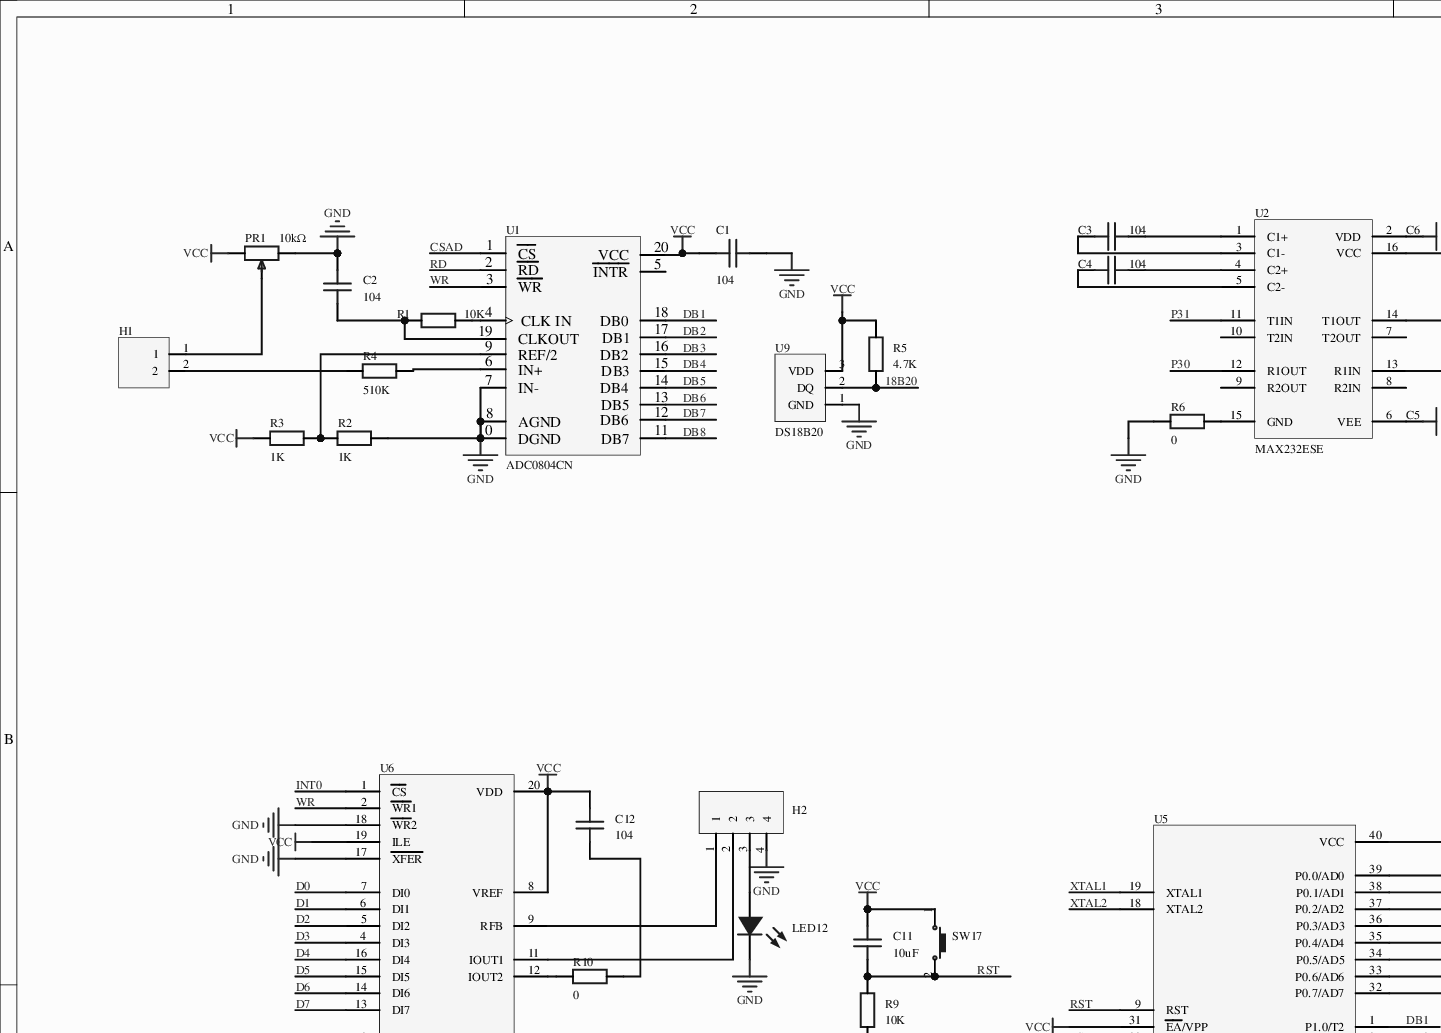
[diagram p0: MISC51981-3.schdoc, top left]
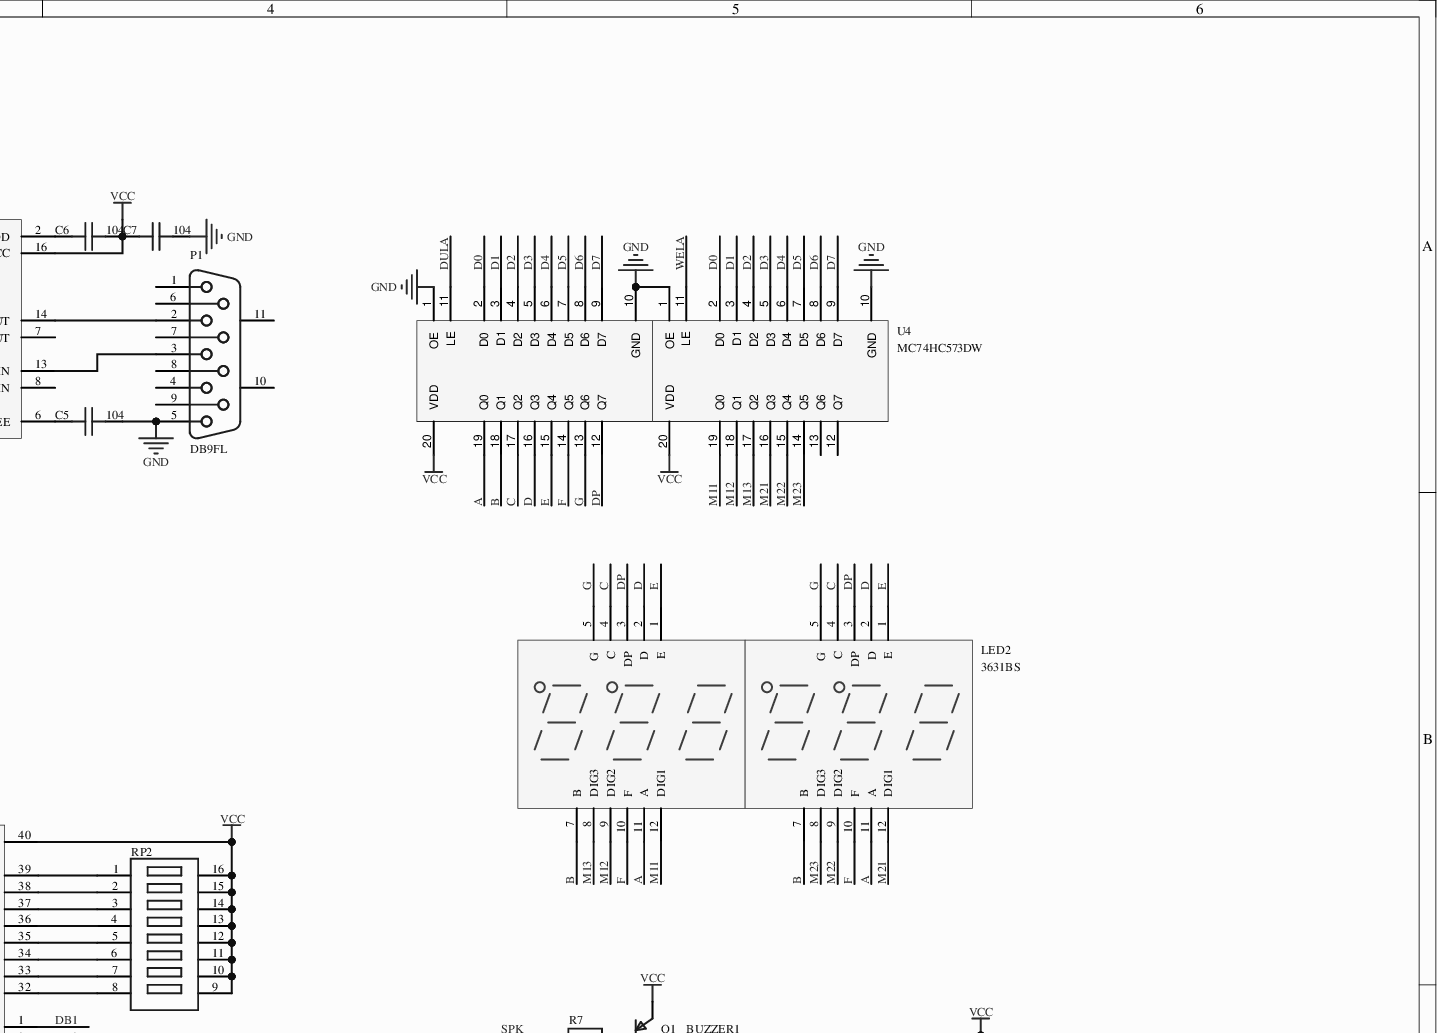
[diagram p1: MISC51981-3.schdoc, top right]
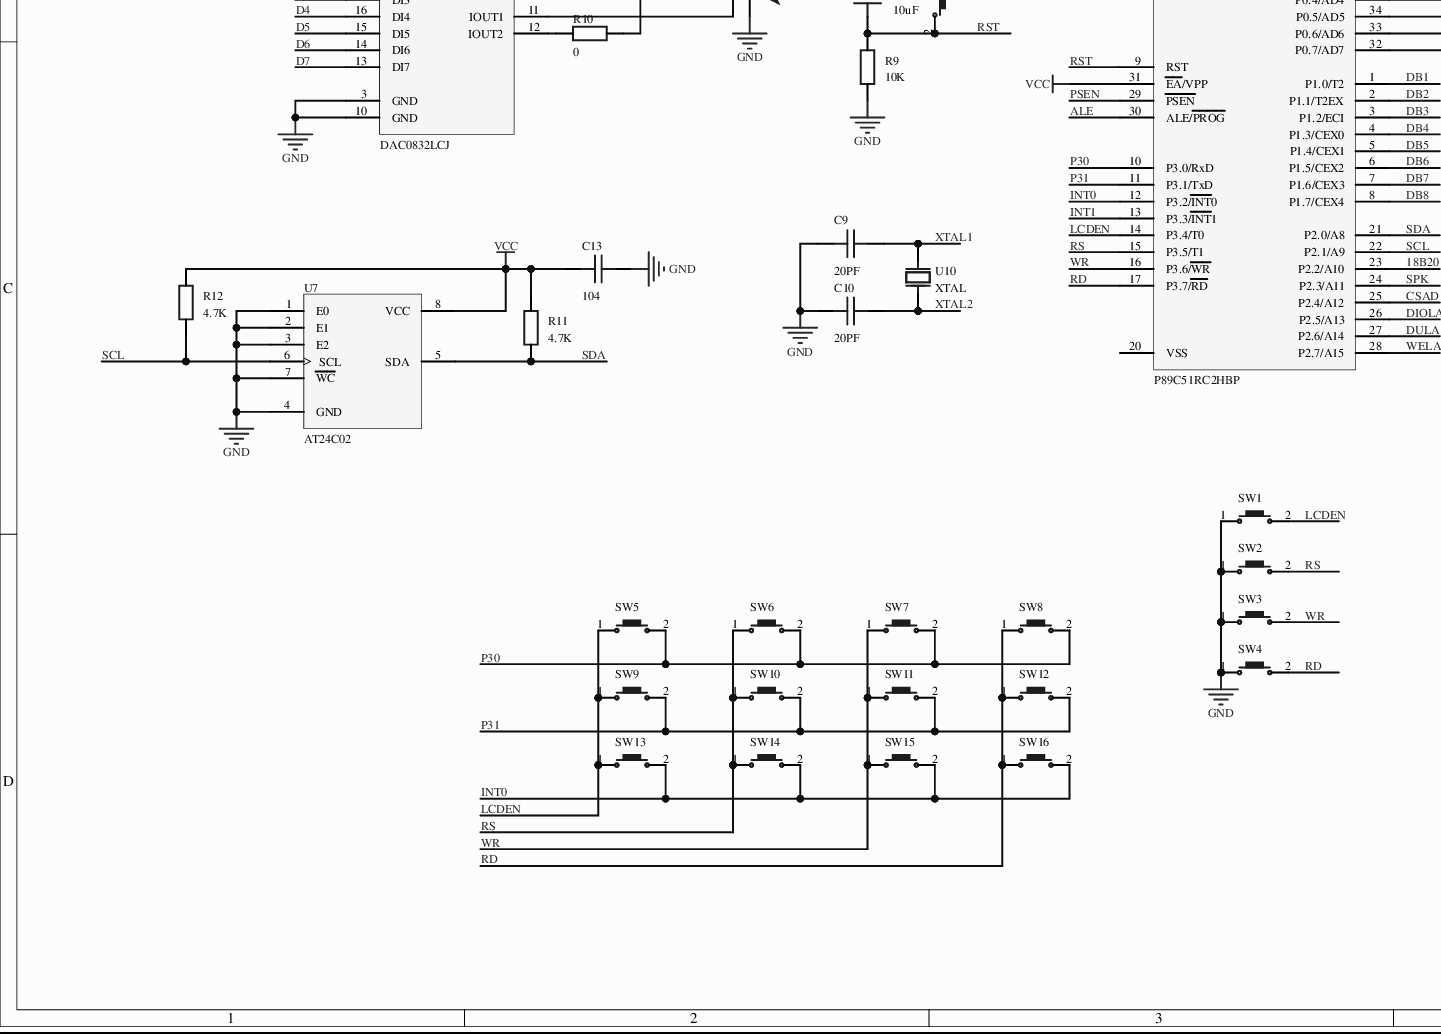
[diagram p2: MISC51981-3.schdoc, bottom left]
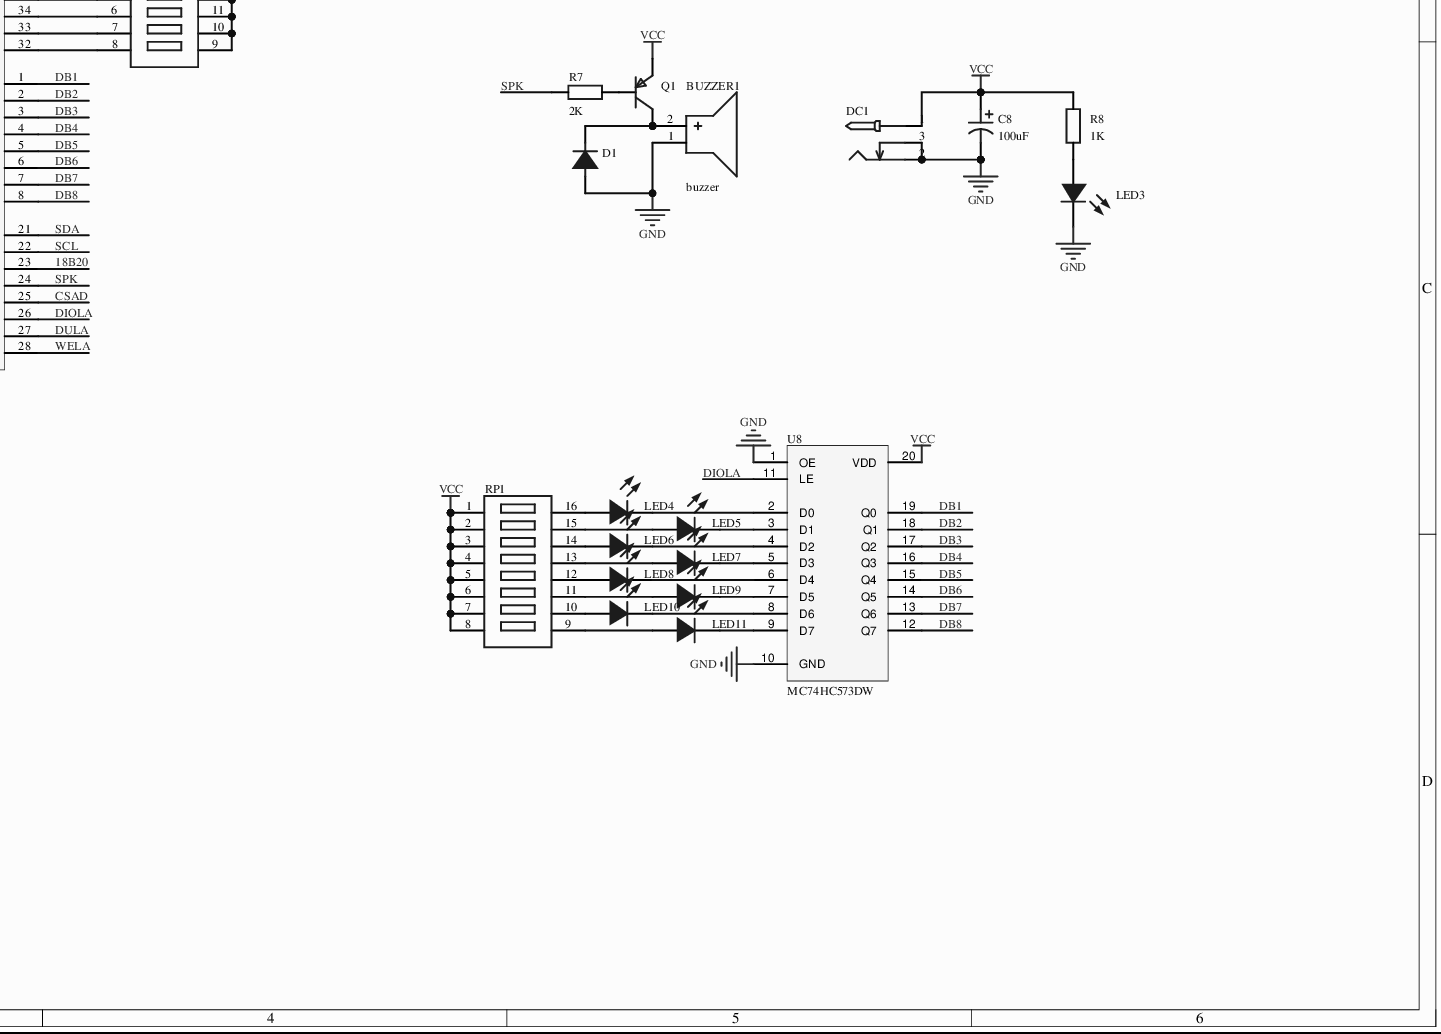
[diagram p3: MISC51981-3.schdoc, bottom right]
# Altium project MISC51981-2.PrjPcb
1 sheet, 74 parts. Net scope: global (net labels, ports and power ports of the same name join across sheets).
Board file: MISC51981.pcbdoc

## Sheet MISC51981-3.schdoc
size 420 x 297 mm; Version: V1.0; @Project Name: MISC51981; @Update Date: 2026-09-29; @Create Date: 2026-09-29; @Board Name: MISC51981; @Create Time: 10:53:11; @Page Count: 1; @Page No: 1; @Schematic Name: MISC51981; @Update Time: 10:53:11; Size: A4

### Parts
BUZZER1  buzzer  [BUZ-TH_BD12.0-P6.00-D0.9-RD]
C1  104  [C0603]
C2  104  [C0603]
C3  104  [C0603]
C4  104  [C0603]
C5  104  [C0603]
C6  104  [C0603]
C7  104  [C0603]
C8  100uF  [CAP-TH_BD5.0-P2.00-D0.8-FD-10UF50VC110GL]
C9  20PF  [C0603]
C10  20PF  [C0603]
C11  10uF  [C0603]
C12  104  [C0603]
C13  104  [C0603]
D1  (no value)  [DO_1N4007]
DC1  (no value)  [DC-005_2.5]
H1  (no value)  [HDR-TH_2P-P2.54-V-M-1]
H2  (no value)  [HDR-TH_4P-P2.54-V-M]
LED1  3631BS  [LED-SEG-TH_11P-L37.5-W19.0-P2.54-LS15.2-BL_1]
LED2  3631BS  [LED-SEG-TH_11P-L37.5-W19.0-P2.54-LS15.2-BL_1]
LED3  (no value)  [LED_0603]
LED4  (no value)  [LED_0603]
LED5  (no value)  [LED_0603]
LED6  (no value)  [LED_0603]
LED7  (no value)  [LED_0603]
LED8  (no value)  [LED_0603]
LED9  (no value)  [LED_0603]
LED10  (no value)  [LED_0603]
LED11  (no value)  [LED_0603]
LED12  (no value)  [LED_0603]
P1  DB9FL  [DB9-TH_DB9F]
PR1  10kΩ  [R_3296]
Q1  (no value)  [S8550P_TO-92]
R1  10K  [R0603]
R2  1K  [R0603]
R3  1K  [R0603]
R4  510K  [R0603]
R5  4.7K  [R0603]
R6  0  [R0603]
R7  2K  [R0603]
R8  1K  [R0603]
R9  10K  [R0603]
R10  0  [R0603]
R11  4.7K  [R0603]
R12  4.7K  [R0603]
RP1  (no value)  [DIP-16_L20.3-W10.2-P2.54-LS7.6-BL]
RP2  (no value)  [DIP-16_L20.3-W10.2-P2.54-LS7.6-BL]
SW1  (no value)  [Key_SMD_3x4x2]
SW2  (no value)  [Key_SMD_3x4x2]
SW3  (no value)  [Key_SMD_3x4x2]
SW4  (no value)  [Key_SMD_3x4x2]
SW5  (no value)  [Key_SMD_3x4x2]
SW6  (no value)  [Key_SMD_3x4x2]
SW7  (no value)  [Key_SMD_3x4x2]
SW8  (no value)  [Key_SMD_3x4x2]
SW9  (no value)  [Key_SMD_3x4x2]
SW10  (no value)  [Key_SMD_3x4x2]
SW11  (no value)  [Key_SMD_3x4x2]
SW12  (no value)  [Key_SMD_3x4x2]
SW13  (no value)  [Key_SMD_3x4x2]
SW14  (no value)  [Key_SMD_3x4x2]
SW15  (no value)  [Key_SMD_3x4x2]
SW16  (no value)  [Key_SMD_3x4x2]
SW17  (no value)  [Key_SMD_3x4x2]
U1  ADC0804CN  [ADC0804CN]
U2  MAX232ESE
U3  MC74HC573DW  (value not drawn)
U4  MC74HC573DW
U5  P89C51RC2HBP
U6  DAC0832LCJ  [J20A]
U7  AT24C02
U8  MC74HC573DW
U9  DS18B20  [TO-92-3_L4.9-W3.7-P1.27-L]
U10  Manufacturer: XTAL  [osc-smd_l3.2-w1.5]  (hidden comment: 32768/10ppm/12.5pF)

### Nets
GND: BUZZER1.1(-) C1.2 C2.2 C5.1 C7.1 C8.2 C9.1 C10.1 C13.2 D1.2(A) DC1.2 DC1.3 H2.4 LED3.1(C) LED12.1(C) P1.5 PR1.3 R2.2 R6.1 R9.1 SW1.1 SW2.1 SW3.1 SW4.1 U1.7(IN-) U1.8(AGND) U1.10(DGND) U3.1(OE) U3.10(GND) U4.1(OE) U4.10(GND) U6.3(GND) U6.10(GND) U6.17(~{XFER}) U6.18(~{WR}2) U7.1(E0) U7.2(E1) U7.3(E2) U7.4(GND) U7.7(~{WC}) U8.1(OE) U8.10(GND) U9.1(GND)
VCC: C1.1 C6.1 C7.2 C8.1 C11.2 C12.2 C13.1 DC1.1 PR1.1 Q1.1(E) R3.1 R5.2 R8.2 R11.2 R12.2 RP1.1 RP1.2 RP1.3 RP1.4 RP1.5 RP1.6 RP1.7 RP1.8 RP2.9 RP2.10 RP2.11 RP2.12 RP2.13 RP2.14 RP2.15 RP2.16 SW17.1 U1.20(VCC) U2.16(VCC) U3.20(VDD) U4.20(VDD) U5.31(~{EA}/VPP) U5.40(VCC) U6.8(VREF) U6.19(ILE) U6.20(VDD) U7.8(VCC) U8.20(VDD) U9.3(VDD)
18B20: R5.1 U5.23(P2.2/A10) U9.2(DQ)
A: LED1.11(A) LED2.11(A) U3.19(Q0)
ALE: U5.30(ALE/~{PROG})
B: LED1.7(B) LED2.7(B) U3.18(Q1)
C: LED1.4(C) LED2.4(C) U3.17(Q2)
CSAD: U1.1(~{CS}) U5.25(P2.4/A12)
D: LED1.2(D) LED2.2(D) U3.16(Q3)
D0: U3.2(D0) U4.2(D0) U6.7(DI0)
D1: U3.3(D1) U4.3(D1) U6.6(DI1)
D2: U3.4(D2) U4.4(D2) U6.5(DI2)
D3: U3.5(D3) U4.5(D3) U6.4(DI3)
D4: U3.6(D4) U4.6(D4) U6.16(DI4)
D5: U3.7(D5) U4.7(D5) U6.15(DI5)
D6: U3.8(D6) U4.8(D6) U6.14(DI6)
D7: U3.9(D7) U4.9(D7) U6.13(DI7)
DB1: U1.18(DB0) U5.1(P1.0/T2) U8.19(Q0)
DB2: U1.17(DB1) U5.2(P1.1/T2EX) U8.18(Q1)
DB3: U1.16(DB2) U5.3(P1.2/ECI) U8.17(Q2)
DB4: U1.15(DB3) U5.4(P1.3/CEX0) U8.16(Q3)
DB5: U1.14(DB4) U5.5(P1.4/CEX1) U8.15(Q4)
DB6: U1.13(DB5) U5.6(P1.5/CEX2) U8.14(Q5)
DB7: U1.12(DB6) U5.7(P1.6/CEX3) U8.13(Q6)
DB8: U1.11(DB7) U5.8(P1.7/CEX4) U8.12(Q7)
DIOLA: U5.26(P2.5/A13) U8.11(LE)
DP: LED1.3(DP) LED2.3(DP) U3.12(Q7)
DULA: U3.11(LE) U5.27(P2.6/A14)
E: LED1.1(E) LED2.1(E) U3.15(Q4)
F: LED1.10(F) LED2.10(F) U3.14(Q5)
G: LED1.5(G) LED2.5(G) U3.13(Q6)
INT0: SW13.2 SW14.2 SW15.2 SW16.2 U5.12(P3.2/~{INT}0) U6.1(~{CS})
INT1: U5.13(P3.3/~{INT}1)
LCDEN: SW1.2 SW5.1 SW9.1 SW13.1 U5.14(P3.4/T0)
M11: LED1.12(DIG1) U4.19(Q0)
M12: LED1.9(DIG2) U4.18(Q1)
M13: LED1.8(DIG3) U4.17(Q2)
M21: LED2.12(DIG1) U4.16(Q3)
M22: LED2.9(DIG2) U4.15(Q4)
M23: LED2.8(DIG3) U4.14(Q5)
P30: SW5.2 SW6.2 SW7.2 SW8.2 U2.12(R1OUT) U5.10(P3.0/RxD)
P31: SW9.2 SW10.2 SW11.2 SW12.2 U2.11(T1IN) U5.11(P3.1/TxD)
PSEN: U5.29(~{PSEN})
RD: SW4.2 SW8.1 SW12.1 SW16.1 U1.2(~{RD}) U5.17(P3.7/~{RD})
RS: SW2.2 SW6.1 SW10.1 SW14.1 U5.15(P3.5/T1)
RST: C11.1 R9.2 SW17.2 U5.9(RST)
SCL: R12.1 U5.22(P2.1/A9) U7.6(SCL)
SDA: R11.1 U5.21(P2.0/A8) U7.5(SDA)
SPK: R7.1 U5.24(P2.3/A11)
WELA: U4.11(LE) U5.28(P2.7/A15)
WR: SW3.2 SW7.1 SW11.1 SW15.1 U1.3(~{WR}) U5.16(P3.6/~{WR}) U6.2(~{WR}1)
XTAL1: C9.2 U5.19(XTAL1) U10.2(OSC2)
XTAL2: C10.2 U5.18(XTAL2) U10.1(OSC1)
NetBUZZER1_2: BUZZER1.2(+) D1.1(K) Q1.3(C)
NetC2_1: C2.1 R1.1 U1.19(CLKOUT)
NetC3_1: C3.1 U2.1(C1+)
NetC3_2: C3.2 U2.3(C1-)
NetC4_1: C4.1 U2.4(C2+)
NetC4_2: C4.2 U2.5(C2-)
NetC5_2: C5.2 U2.6(VEE)
NetC6_2: C6.2 U2.2(VDD)
NetC12_1: C12.1 R10.2
NetH1_1: H1.1 PR1.2
NetH1_2: H1.2 R4.1
NetH2_1: H2.1 U6.9(RFB)
NetH2_2: H2.2 U6.11(IOUT1)
NetH2_3: H2.3 LED12.2(A)
NetLED3_2: LED3.2(A) R8.1
NetLED4_1: LED4.1(C) U8.2(D0)
NetLED4_2: LED4.2(A) RP1.16
NetLED5_1: LED5.1(C) U8.3(D1)
NetLED5_2: LED5.2(A) RP1.15
NetLED6_1: LED6.1(C) U8.4(D2)
NetLED6_2: LED6.2(A) RP1.14
NetLED7_1: LED7.1(C) U8.5(D3)
NetLED7_2: LED7.2(A) RP1.13
NetLED8_1: LED8.1(C) U8.6(D4)
NetLED8_2: LED8.2(A) RP1.12
NetLED9_1: LED9.1(C) U8.7(D5)
NetLED9_2: LED9.2(A) RP1.11
NetLED10_1: LED10.1(C) U8.8(D6)
NetLED10_2: LED10.2(A) RP1.10
NetLED11_1: LED11.1(C) U8.9(D7)
NetLED11_2: LED11.2(A) RP1.9
NetP1_2: P1.2 U2.14(T1OUT)
NetP1_3: P1.3 U2.13(R1IN)
NetQ1_2: Q1.2(B) R7.2
NetR1_2: R1.2 U1.4(CLK_IN)
NetR2_1: R2.1 R3.2 U1.9(REF/2)
NetR4_2: R4.2 U1.6(IN+)
NetR6_2: R6.2 U2.15(GND)
NetR10_1: R10.1 U6.12(IOUT2)
NetRP2_1: RP2.1 U5.39(P0.0/AD0)
NetRP2_2: RP2.2 U5.38(P0.1/AD1)
NetRP2_3: RP2.3 U5.37(P0.2/AD2)
NetRP2_4: RP2.4 U5.36(P0.3/AD3)
NetRP2_5: RP2.5 U5.35(P0.4/AD4)
NetRP2_6: RP2.6 U5.34(P0.5/AD5)
NetRP2_7: RP2.7 U5.33(P0.6/AD6)
NetRP2_8: RP2.8 U5.32(P0.7/AD7)

Not connected (* = marked no-connect by the designer): P1 1* 4* 6* 7* 8* 9* 10(MH1)* 11(MH2)*; U1 5(~{INTR})*; U2 7(T2OUT)* 8(R2IN)* 9(R2OUT)* 10(T2IN)*; U4 12(Q7)* 13(Q6)*; U5 20(VSS)*

### Library data of the parts
BUZZER1 = buzzer: AddInBom: yes; ModelId: af17e4151ed84fc2a628230bf23763630819f05c4eef4c71ace90d822a990e87; ModelTransform: 472.44,472.176,0,270,0,0,0,0,-196.85; Symbol: BUZZER; Device: buzzer; FootprintName: BUZ-TH_BD12.0-P6.00-D0.9-RD; LCSC Part Name: buzzer; SupplierPart: C9900014030; ManufacturerPart: buzzer; Supplier Footprint: buzzer; JLCPCB Part Class: Extended Part; Supplier: LCSC; ConvertToPcb: yes; ModelName: BUZ-TH_BD12.0-P6.00-D0.9-RD
C1-C7 C9-C13 = CAP_0603: Symbol: Capacitance; ConvertToPcb: yes; ModelId: ac125912035d415993ca9572d50418b10819f05c4eef4c71ace90d822a990e87; ModelName: C0603_L1.6-W0.8-H0.8; ModelTransform: 62.992,31.496,0,0,0,0,0,0,0; Device: CAP_0603; FootprintName: C0603; AddInBom: yes; Supplier Footprint: 0603
  C1-C7 C12 C13: Value: 104
  C9 C10: Value: 20PF
  C11: Value: 10uF
C8 = 10UF50VC110GL: 容值:10uF;精度:±20%;额定电压:50V;纹波电流:120mA@100KHz;等效串联电阻(ESR):1.6Ω;; Manufacturer: Econd(米朗电子); AddInBom: yes; ModelId: b35ab6b0460c4c43a629d91cfc2b58780819f05c4eef4c71ace90d822a990e87; ModelTransform: 196.85,196.85,0,0,0,0,0,0,-196.85; Tolerance: ±20%; Voltage Rating: 50V; Equivalent Series Resistance(ESR): 1.6Ω; Pin Spacing: 2mm; Lifetime: 5000hrs@105℃; Symbol: 10UF50VC110GL; Device: 10UF50VC110GL; Value: 100uF; FootprintName: CAP-TH_BD5.0-P2.00-D0.8-FD-10UF50VC110GL; LCSC Part Name: 10uF ±20% 50V; ManufacturerPart: 10UF50VC110GL; Supplier Footprint: 插件,D5xL11mm; JLCPCB Part Class: Extended Part; Datasheet: https://item.szlcsc.com/datasheet/10UF50VC110GL/49031974.html; Supplier: LCSC; ConvertToPcb: yes; ModelName: CAP-TH_BD5.0-P2.00-D0.8-FD-10UF50VC110GL; Ripple Current: 120mA@100KHz; Diameter: 5mm; Height - Seated (Max): 11mm; Operating Temperature: -40℃~+105℃
D1 = D_1N4007A: AddInBom: yes; ModelId: 6de1e9b71a0d4751b4e9df530304c1a30819f05c4eef4c71ace90d822a990e87; ModelName: DO-41_D2.4-L4.7-P8.70; ModelTransform: 373.9,94.4,232.29,0,0,0,0,0,-140; Symbol: D_1N4007; Device: D_1N4007A; FootprintName: DO_1N4007; Supplier Footprint: DO-41; ConvertToPcb: yes
DC1 = DC-005_2.5: ConvertToPcb: yes; ModelId: f168fe383f964e0ea2af0127ff6ac7b40819f05c4eef4c71ace90d822a990e87; ModelName: DC-IN-TH_DC005; ModelTransform: 366.14,553.15,590.55,90,0,0,137.8,-11.81,-157.48; Symbol: DC-005_2.5; Device: DC-005_2.5; FootprintName: DC-005_2.5; AddInBom: yes; Supplier Footprint: 插件
H1 = HDR-M_2.54_1x2P: Symbol: 210S-1*2P L=11.6MMGold-plated black; ConvertToPcb: yes; ModelId: 79b2e9f2d70a4d68a1b7098f27c6d4c50819f05c4eef4c71ace90d822a990e87; ModelName: HDR-M-2.54_1x2; ModelTransform: 200,100,0,0,0,0,0,0,-118.11; Device: HDR-M_2.54_1x2P; FootprintName: HDR-TH_2P-P2.54-V-M-1; AddInBom: yes; SupplierPart: C124375; Supplier Footprint: 插件
H2 = HDR-M_2.54_1x4P: Symbol: PZ254V-11-04P; ConvertToPcb: yes; ModelId: 112f4d05e8d64e99ab9a333894bea4f90819f05c4eef4c71ace90d822a990e87; ModelName: HDR-TH_4P-P2.54-M-LI-1X4P; ModelTransform: 399.999,104.7242,0,0,0,0,0,0,-118.11; Device: HDR-M_2.54_1x4P; FootprintName: HDR-TH_4P-P2.54-V-M; AddInBom: yes; SupplierPart: C492403; Supplier Footprint: 插件
LED1 LED2 = 3631BS: 数码管位数:3位;发光颜色:蓝色;LED极性:共阳极;数字/字母大小(英寸):0.56;; Manufacturer: 志浩; Number of Characters: 3位; Luminous Color: 蓝色; LED Polarity: 共阳极; Digit/Alpha Size(inch): 0.56; 3D Model: f54e6f5f8ebd42c59fa542745733582317bf92a994fa409e84525e65b42a2577; 3D Model Transform: 1476.375,748.424,0,0,0,0,0,0,-157.48; AddInBom: yes; Symbol: 3631BS; Device: 3631BS; LCSC Part Name: 3位0.56英寸 蓝光共阳 数码管; Supplier Part: C2938341; Manufacturer Part: 3631BS; Supplier Footprint: 插件; JLCPCB Part Class: 扩展库; Datasheet: https://atta.szlcsc.com/upload/public/pdf/source/20220104/5C2FBAA78B63B49D128F0D9B62C0A18B.pdf; Supplier: LCSC; FootprintName: LED-SEG-TH_11P-L37.5-W19.0-P2.54-LS15.2-BL_1; ConvertToPcb: yes; ModelName: LED-SEG-TH_11P-L37.5-W19.0-P2.54-LS15.2-BL_1
LED3-LED12 = LED_0603-B: Symbol: LED_B; Convert to PCB: yes; 3D Model: eb8d964598f24248affda46f619856c50819f05c4eef4c71ace90d822a990e87; 3D Model Transform: 63.1,31.6,23.7,0,0,0,0,0,0; ModelName: LED-0603_B; Device: LED_0603-B; Add into BOM: yes; Supplier Footprint: 0603; FootprintName: LED_0603
P1 = DB9FL: AddInBom: yes; ModelId: fd27160e2e724a89a2372c6f814078df314da64f82a2492c9607ff1f6bb3435e; ModelName: DB9-TH_DB9-H-F_C2888345; ModelTransform: 1212.596,700.786,0,0,0,0,0,-230.315,-177.165; Symbol: DB9FL; Device: DB9FL; FootprintName: DB9-TH_DB9F; LCSC Part Name: DB9FL; SupplierPart: C9900001807; ManufacturerPart: DB9FL; Supplier Footprint: DConnector9; JLCPCB Part Class: 扩展库; Supplier: LCSC; ConvertToPcb: yes
PR1 = R_3296: ConvertToPcb: yes; ModelId: b182808559bb43bda9e7de64b64134cb0819f05c4eef4c71ace90d822a990e87; ModelName: 3296W; ModelTransform: 373.98,188.96,590.49,180,0,0,0,0,-140; Symbol: R_3296; Device: R_3296; FootprintName: R_3296; AddInBom: yes; Supplier Footprint: 直插; Value: 10kΩ
Q1 = S8550_TO_PNP: ConvertToPcb: yes; ModelId: aafe8e06f2154e7c93506efd0d6632dd0819f05c4eef4c71ace90d822a990e87; ModelName: TO-92-3_L4.9-W3.7-P1.27-L; ModelTransform: 180.78,141.44,417.3,0,0,0,0,0,-200; Symbol: S8550_TO_PNP; Device: S8550_TO_PNP; FootprintName: S8550P_TO-92; AddInBom: yes; Supplier Footprint: TO-92
R1-R12 = Res_0603: Symbol: 电阻; ConvertToPcb: yes; ModelId: fc143cca1e79419f9cd78b61e9279f080819f05c4eef4c71ace90d822a990e87; ModelTransform: 31.8897,63.7794,0,90,0,0,0,0,0; Device: Res_0603; FootprintName: R0603; AddInBom: yes; Supplier Footprint: 0603; ModelName: R0603
  R1 R9: Value: 10K
  R2 R3 R8: Value: 1K
  R4: Value: 510K
  R5 R11 R12: Value: 4.7K
  R6 R10: Value: 0
  R7: Value: 2K
RP1 RP2 = paizu: AddInBom: yes; ModelId: b73b726218474b419f7d257eb9cc4370d07147df35bb4ee1ae33039552c243e2; ModelName: DIP-16_L20.3-W10.2-P2.54-LS7.6-BL-1; ModelTransform: 799.998,399.999,0,0,0,0,0,0,-118.11; Symbol: paizu; Device: paizu; ConvertToPcb: yes; FootprintName: DIP-16_L20.3-W10.2-P2.54-LS7.6-BL
SW1-SW17 = Key_SMD_3x4x2: Symbol: 轻触按键x2; ConvertToPcb: yes; ModelId: 63599cce708d48afbce1b0db003544770819f05c4eef4c71ace90d822a990e87; ModelName: SW-SMD_L4.0-W2.9-H2-LS5.0; ModelTransform: 196.85,114.17,79.13,0,0,0,0,0,0; Device: Key_SMD_3x4x2; FootprintName: Key_SMD_3x4x2; AddInBom: yes; Supplier Footprint: SMD
U1 = ADC0804CN: AddInBom: yes; Symbol: ADC0804CN; Device: ADC0804CN; FootprintName: ADC0804CN; ConvertToPcb: yes
U2 = MAX232ESE: RS232; Package1: SOIC-16_150mil; AddInBom: yes; Symbol: MAX232ESE; Device: MAX232ESE; ComponentLink1Description: 供应商链接; ComponentLink1URL: http://www.szlcsc.com/product/details_27608.html; Supplier: LC; SuppliersPartNumber: C26860; Footprint Name: LC-SOIC-16_150mil; ConvertToPcb: yes
U3 U4 U8 = MC74HC573DW: ConvertToPcb: yes; Symbol: MC74HC573DW; Device: MC74HC573DW; AddInBom: yes
U5 = P89C51RC2HBP: AddInBom: yes; Symbol: P89C51RC2HBP; Device: P89C51RC2HBP; ConvertToPcb: yes
U6 = DAC0832LCJ: ComponentAvailability: Obsolete; AddInBom: yes; Symbol: DAC0832LCJ; Device: DAC0832LCJ; Published: 15-Apr-2002; LatestRevisionDate: 06-Jun-2005; LatestRevisionNote: Stylized 3D Model Added.; DatasheetVersion: May-1999; PackageVersion: 2000; PackageReference: J20A; PackageDescription: DIP; 20 Leads; Row Spacing 7.62 mm; Pitch 2.54 mm; Code_JEDEC: MS-015-AE; ComponentLink1Description: Manufacturer Link; ComponentLink1URL: http://www.national.com/; ComponentLink2Description: Datasheet; ComponentLink2URL: http://www.national.com/ds.cgi/DA/DAC0830.pdf; ComponentLink3Description: Discontinuation Notice; ComponentLink3URL: http://www.national.com/obs/obsolescence.txt; ComponentLink4Description: URL Link1; ComponentLink4URL: http://www.national.com/pf/DA/DAC0832.html; ConvertToPcb: yes; FootprintName: J20A; Publisher: Altium Limited
U7 = M24C02BN6: AddInBom: yes; Origin Footprint 2: PSDIP8A; Origin Footprint 3: SOP8_L; Origin Footprint 4: SOP8_N; Origin Footprint 5: AT24CB; Origin Footprint 6: DIP8; Symbol: M24C02BN6; Device: M24C02BN6; ConvertToPcb: yes; Published: 24-Aug-2001; LatestRevisionDate: 06-Jun-2005; LatestRevisionNote: Stylized 3D Model Added.; DatasheetVersion: Sep-1999; PackageVersion: Jun-1998; PackageReference: PSDIP8A; PackageDescription: DIP; 8 Leads; Row Spacing 7.62 mm; Pitch 2.54 mm; ComponentLink1Description: Manufacturer Link; ComponentLink1URL: http://www.st.com/; ComponentLink2Description: Datasheet; ComponentLink2URL: http://www.st.com/stonline/products/literature/ds/5067/m24c01-r.pdf; Publisher: Altium Limited
U9 = DS18B20: Manufacturer: Youtai Semiconductor Co., Ltd.; AddInBom: yes; ModelId: aafe8e06f2154e7c93506efd0d6632ddc675cafc06334f02bb6e99fe0a86729f; Symbol: DS18B20; Device: DS18B20; FootprintName: TO-92-3_L4.9-W3.7-P1.27-L; Supplier: LCSC; SupplierPart: C376006; ManufacturerPart: DS18B20; JLCPCB Part Class: Extended Part; ConvertToPcb: yes; ModelName: TO-92-3_L4.9-W3.7-P1.27-L
U10 = 32768/10ppm/12.5pF: AddInBom: yes; ModelId: 2dd241c0893b4675b8def6f6998a8251343fa624c39949f9abdc5569de48b688; ModelName: OSC-SMD_L3.2-W1.5-H0.8; ModelTransform: 125.984,59.055,0,0,0,0,0,0,0; Symbol: 32768/10ppm/12.5pf; Device: 32768/10ppm/12.5pF; FootprintName: osc-smd_l3.2-w1.5; LCSC Part Name: 32768/10ppm/12.5pF; SupplierPart: C9900093280; ManufacturerPart: 32768/10ppm/12.5pF; Supplier Footprint: XTAL3215; JLCPCB Part Class: 扩展库; Supplier: LCSC; ConvertToPcb: yes